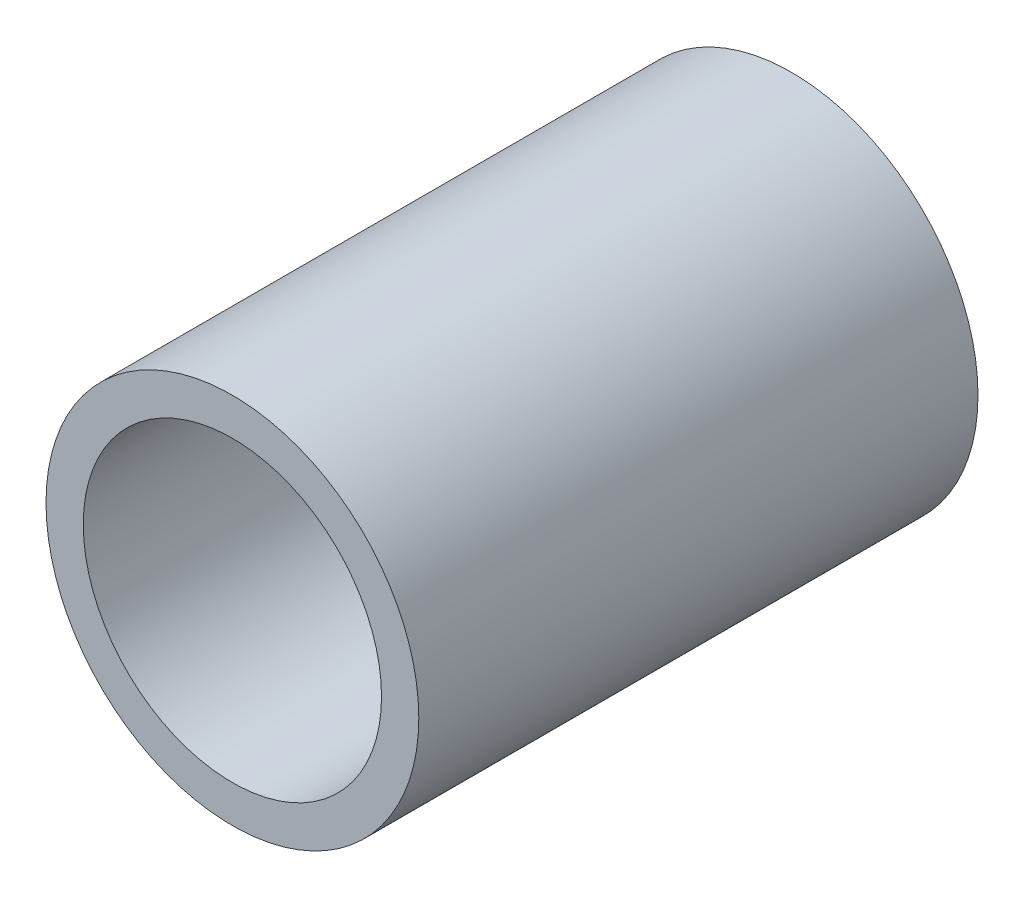
SolidWorks part; units mm, degrees
material "PP 共聚物"
ref_plane "前视基准面" through (0, 0, 0) normal (0, 0, 1) x (1, 0, 0)
ref_plane "上视基准面" through (0, 0, 0) normal (0, 1, 0) x (1, 0, 0)
ref_plane "右视基准面" through (0, 0, 0) normal (1, 0, 0) x (0, 0, -1)
sketch "草图1" plane through (0, 0, 0) normal (0, 0, 1) x (1, 0, 0)
  circle A0 centre (0, 0) radius 10
  dimension "D1" = 20
extrude "拉伸-薄壁1" add sketch "草图1" along normal blind 30 thin thin type one direction reverse wall 2
